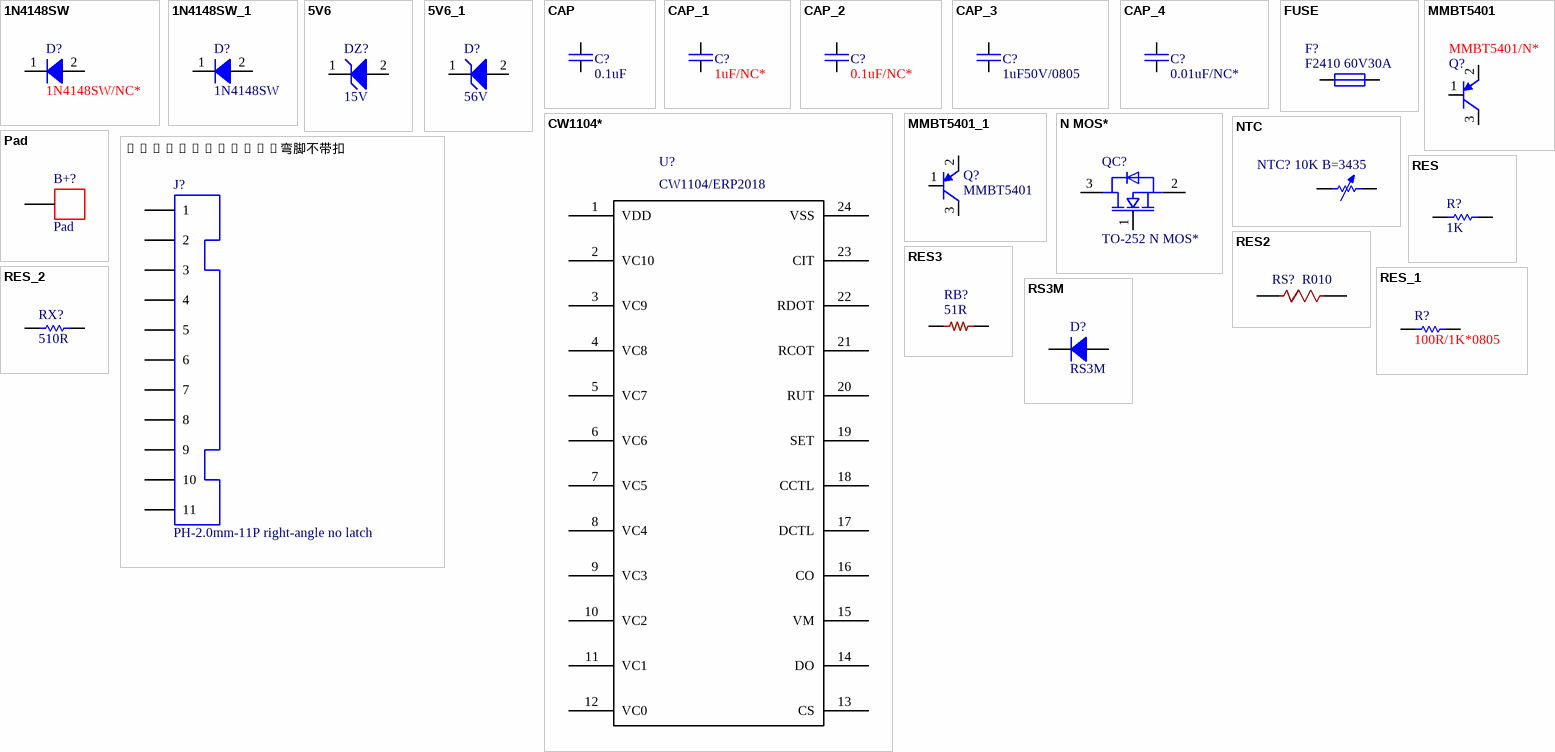
[diagram p0: symbols 1N4148SW to RS3M]
# Altium schematic symbol library MISC84401-4.SchLib: 23 symbols
Pins are listed as number, name and electrical type; pins without a type are passive.


## 1N4148SW
designator D?, comment 1N4148SW/NC*
SMD diode
footprint SOD123 (SMD diode)
footprint SOD323 (SMD diode)
pins: 1 A, 2 K

## 1N4148SW_1
designator D?, comment 1N4148SW
SMD diode
footprint SOD123 (SMD diode)
footprint SOD323 (SMD diode)
pins: 1 A, 2 K

## 5V6
designator DZ?, comment 15V
SMD Zener diode
footprint SOD323 (SMD diode)
footprint SOD123 (SMD diode)
pins: 1 A, 2 K

## 5V6_1
designator D?, comment 56V
SMD Zener diode
footprint SOD323 (SMD diode)
footprint SOD123 (SMD diode)
pins: 1 A, 2 K

## CAP
designator C?, comment 0.1uF
SMD capacitor
footprint C0402A (SMD capacitor)
footprint C0603A (SMD capacitor)
footprint C0402L (SMD resistor)
footprint C0805A (SMD capacitor)
footprint C1206A (SMD capacitor)
footprint C0603L (SMD J capacitor)
footprint C0805L (SMD capacitor)
pins: 1, 2

## CAP_1
designator C?, comment 1uF/NC*
SMD capacitor
footprint C0402A (SMD capacitor)
footprint C0603A (SMD capacitor)
footprint C0402L (SMD resistor)
footprint C0805A (SMD capacitor)
footprint C1206A (SMD capacitor)
footprint C0603L (SMD J capacitor)
footprint C0805L (SMD capacitor)
pins: 1, 2

## CAP_2
designator C?, comment 0.1uF/NC*
SMD capacitor
footprint C0402A (SMD capacitor)
footprint C0603A (SMD capacitor)
footprint C0402L (SMD resistor)
footprint C0805A (SMD capacitor)
footprint C1206A (SMD capacitor)
footprint C0603L (SMD J capacitor)
footprint C0805L (SMD capacitor)
pins: 1, 2

## CAP_3
designator C?, comment 1uF50V/0805
SMD capacitor
footprint C0402A (SMD capacitor)
footprint C0603A (SMD capacitor)
footprint C0402L (SMD resistor)
footprint C0805A (SMD capacitor)
footprint C1206A (SMD capacitor)
footprint C0603L (SMD J capacitor)
footprint C0805L (SMD capacitor)
pins: 1, 2

## CAP_4
designator C?, comment 0.01uF/NC*
SMD capacitor
footprint C0402A (SMD capacitor)
footprint C0603A (SMD capacitor)
footprint C0402L (SMD resistor)
footprint C0805A (SMD capacitor)
footprint C1206A (SMD capacitor)
footprint C0603L (SMD J capacitor)
footprint C0805L (SMD capacitor)
pins: 1, 2

## CW1104*
designator U?, comment CW1104/ERP2018
Cellwise 7-10S battery protection IC
footprint TSSOP-24(pin间距0.635mm) (SMD IC)
pins: 1 VDD, 2 VC10, 3 VC9, 4 VC8, 5 VC7, 6 VC6, 7 VC5, 8 VC4, 9 VC3, 10 VC2, 11 VC1, 12 VC0, 13 CS, 14 DO, 15 VM, 16 CO, 17 DCTL, 18 CCTL, 19 SET, 20 RUT, 21 RCOT, 22 RDOT, 23 CIT, 24 VSS

## FUSE
designator F?, comment F2410 60V30A
footprint R1206A (SMD resistor)
footprint R0603A (SMD resistor)
footprint R0805A (SMD resistor)
footprint F2410 (SMD fuse)
pins: 1, 2

## MMBT5401
designator Q?, comment MMBT5401/N*
SMD transistor
footprint SOT23-3 (SMD IC/MOS*)
footprint SOT23-3L (SMD IMOS)
footprint SOT23-3 (SMD IC/MOS*)
pins: 1 B, 2 E, 3 C

## MMBT5401_1
designator Q?, comment MMBT5401
SMD transistor
footprint SOT23-3 (SMD IC/MOS*)
footprint SOT23-3L (SMD IMOS)
footprint SOT23-3 (SMD IC/MOS*)
pins: 1 B, 2 E, 3 C

## N MOS*
designator QC?, comment TO-252 N MOS*
SMD MOS
footprint TOLL (SMD MOS)
footprint TO-252
footprint TO-252-DFN
pins: 1 G, 2 S, 3 D

## NTC
designator NTC?, comment 10K B=3435
SMD thermistor
footprint R0603A (SMD resistor)
footprint R0402A (SMD resistor)
footprint RT2.3X1-2 (Wire-soldered NTC)
footprint R0603L (SMD resistor)
footprint R0603m (SMD resistor)
footprint RT2.3X1.2-2 (Wire-soldered NTC)
pins: 1, 2

## Pad
designator B+?
Connection pad (non-through-hole)
footprint 3*3
footprint Pad10X8mm
footprint Pad8X6mm
pins: 1

## PH-2.0mm-11P弯脚不带扣
designator J?, comment PH-2.0mm-11P right-angle no latch
Right-angle connector without latch
footprint PH-2.0mm11P弯脚不带扣 (PH-2.0mm11P right-angle connector without latch)
pins: 1, 2, 3, 4, 5, 6, 7, 8, 9, 10, 11

## RES
designator R?, comment 1K
SMD resistor
footprint R0603A (SMD resistor)
footprint R0201A
footprint R0402A (SMD resistor)
footprint R0603m (SMD resistor)
footprint R0805A (SMD resistor)
footprint R0402L (SMD resistor)
footprint RES0603 (CAP0402)
footprint R0603L (SMD resistor)
footprint R0805L (SMD resistor)
footprint R0805M (SMD resistor)
footprint R1206A (SMD resistor)
pins: 1, 2

## RES2
designator RS?, comment R010
SMD alloy resistor
footprint R2512L (SMD resistor)
pins: 1, 2

## RES3
designator RB?, comment 51R
Alloy SMD resistor
footprint R1206A
pins: 1, 2

## RES_1
designator R?, comment 100R/1K*0805
SMD resistor
footprint R0603A (SMD resistor)
footprint R0201A
footprint R0402A (SMD resistor)
footprint R0603m (SMD resistor)
footprint R0805A (SMD resistor)
footprint R0402L (SMD resistor)
footprint RES0603 (CAP0402)
footprint R0603L (SMD resistor)
footprint R0805L (SMD resistor)
footprint R0805M (SMD resistor)
footprint R1206A (SMD resistor)
pins: 1, 2

## RES_2
designator RX?, comment 510R
SMD resistor
footprint R0603A (SMD resistor)
footprint R0201A
footprint R0402A (SMD resistor)
footprint R0603m (SMD resistor)
footprint R0805A (SMD resistor)
footprint R0402L (SMD resistor)
footprint RES0603 (CAP0402)
footprint R0603L (SMD resistor)
footprint R0805L (SMD resistor)
footprint R0805M (SMD resistor)
footprint R1206A (SMD resistor)
pins: 1, 2

## RS3M
designator D?
SMD diode
footprint SMAF
footprint SMB(DO-214AA) (SMD diode)
footprint SMC(DO-214AB) (SMD diode)
pins: 1 A, 2 K